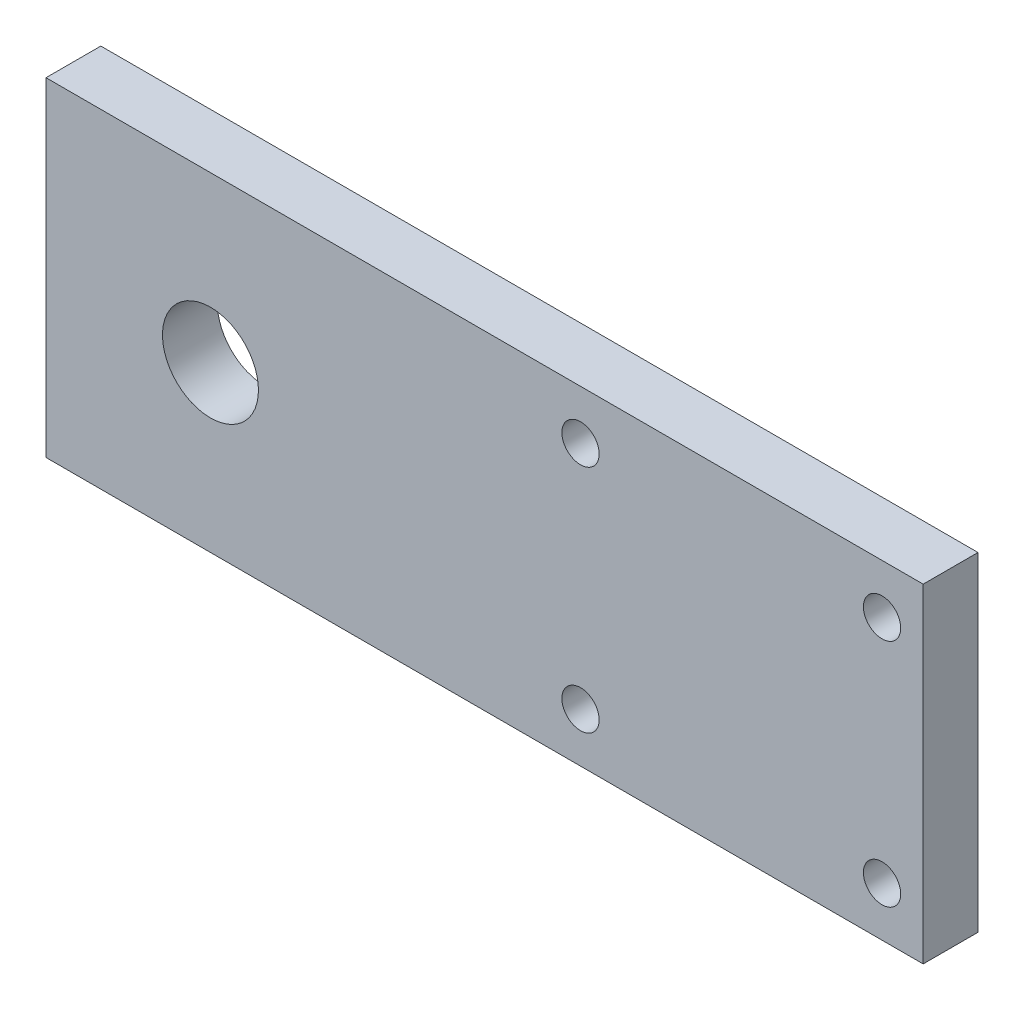
SolidWorks part; units mm, degrees
ref_plane "前视基准面" through (0, 0, 0) normal (0, 0, 1) x (1, 0, 0)
ref_plane "上视基准面" through (0, 0, 0) normal (0, 1, 0) x (1, 0, 0)
ref_plane "右视基准面" through (0, 0, 0) normal (1, 0, 0) x (0, 0, -1)
sketch "草图1" plane through (0, 0, 0) normal (0, 0, 1) x (1, 0, 0)
  line L1 (-80, 30) -> (80, 30)
  line L2 (-80, 30) -> (-80, -30)
  line L3 (-80, -30) -> (80, -30)
  line L4 (80, 30) -> (80, -30)
  line L5 (-80, 30) -> (80, -30) construction
  line L6 (-80, -30) -> (80, 30) construction
  point P0 (0, 0)
  dimension "D1" = 160
  dimension "D2" = 60
extrude "凸台-拉伸1" add sketch "草图1" along normal blind 10
hole_wizard "M20 螺纹孔1" positions "草图2" profile "草图3" tap size "M20" standard "ISO" end condition up to next
sketch "草图2" plane through (0, 0, 10) normal (0, 0, 1) x (1, 0, 0)
  line L0 (-80, 0) -> (80, 0)
  line L1 (-80, 30) -> (-80, -30) construction
  line L2 (80, -30) -> (80, 30) construction
  point P0 (-50, 0)
  dimension "D1" = 30
sketch "草图3" plane through (-50, 0, 10) normal (1, 0, 0) x (0, -1, 0)
  line L0 (0, 0) -> (0, 10)
  line L1 (0, 10) -> (8.75, 10)
  line L2 (8.75, 10) -> (8.75, 0)
  line L5 (8.75, 0) -> (0, 0)
  line L11 (0, -6.35) -> (0, 107.95) construction
  dimension "通孔螺纹孔钻头直径" = 17.5
  dimension "通孔螺纹孔钻头深度" = 10
cosmetic thread "孔螺蚊线1" parameters "D2"=20
hole_wizard "M8 螺纹孔1" positions "草图6" profile "草图7" tap size "M8" standard "ISO" end condition through all
sketch "草图6" plane through (0, 0, 10) normal (0, 0, 1) x (1, 0, 0)
  point P0 (17.5, 21)
  point P3 (72.5, 21)
  point P6 (17.5, -21)
  point P9 (72.5, -21)
sketch "草图7" plane through (17.5, 21, 10) normal (1, 0, 0) x (0, -1, 0)
  line L0 (0, 0) -> (0, 10)
  line L1 (0, 10) -> (3.4, 10)
  line L2 (3.4, 10) -> (3.4, 0)
  line L5 (3.4, 0) -> (0, 0)
  line L11 (0, -6.35) -> (0, 107.95) construction
  dimension "通孔螺纹孔钻头直径" = 6.8
  dimension "通孔螺纹孔钻头深度" = 10
cosmetic thread "孔螺蚊线2" parameters "D2"=8
cosmetic thread "孔螺蚊线3" parameters "D2"=8
cosmetic thread "孔螺蚊线4" parameters "D2"=8
cosmetic thread "孔螺蚊线5" parameters "D2"=8
